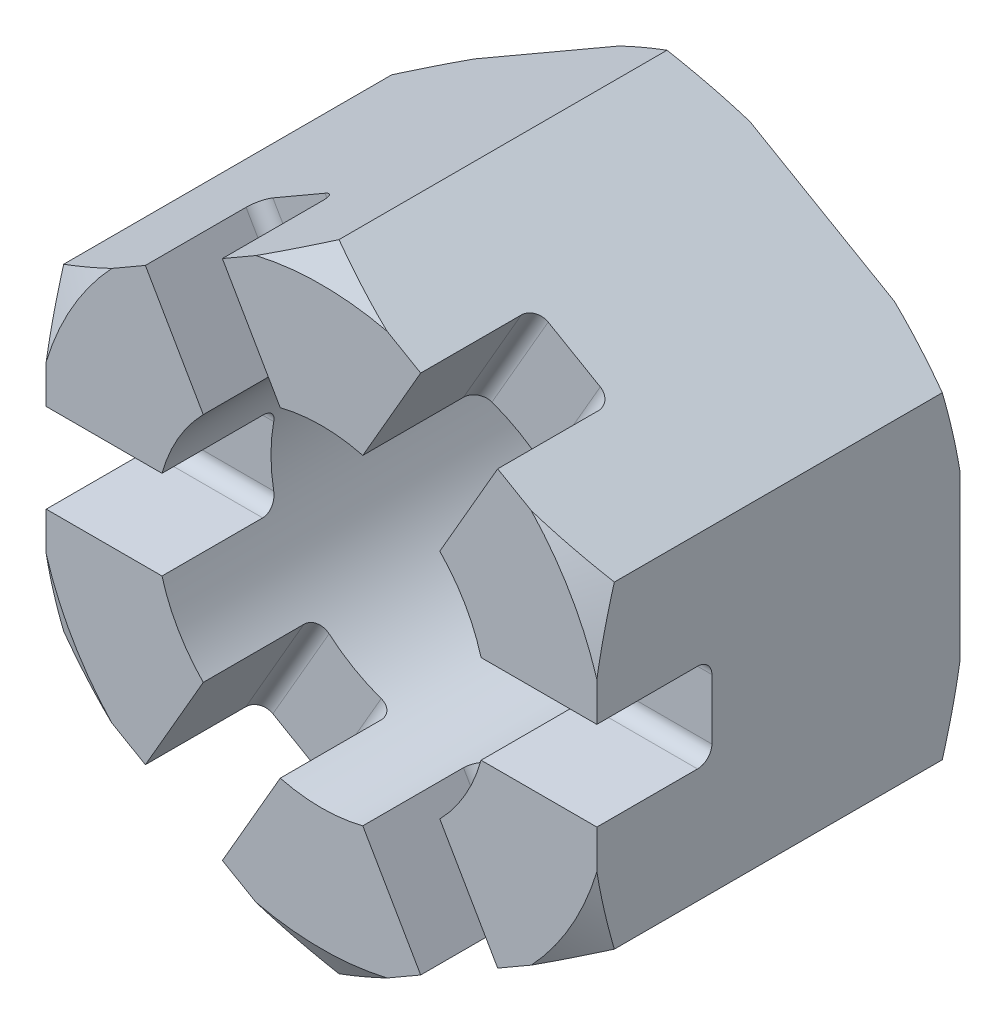
from build123d import *

# Parameters (mm, degrees)
SKETCH_1_R               = 15.835
EXTRUDE_848_DEPTH        = 34.7
SKETCH_2_OUTSIDE_W       = 259.61
SKETCH_2_OUTSIDE_H       = 267.754
SKETCH_2_OUTSIDE_R       = 27.5
CUT_EXTRUDE_1_DEPTH      = 54.111562242
CUT_EXTRUDE_1_DRAFT      = -60
SKETCH_3_OUTSIDE_W       = 259.61
SKETCH_3_OUTSIDE_H       = 267.754
SKETCH_3_OUTSIDE_R       = 27.5
CUT_EXTRUDE_2_DEPTH      = 54.111562242
CUT_EXTRUDE_2_DRAFT      = -60
CUT_EXTRUDE_3_DEPTH      = 70.9965292
PATTERN_CIRCULAR_1_COUNT = 3
CHAMFER_1_SIZE           = 0.576785714


with BuildPart() as part:
    # 草图1 → Extrude 848 (new body)
    with BuildSketch(Plane.XY):
        Polygon((0, 30.395), (-26.322842148, 15.1975), (-26.322842148, -15.1975), (0, -30.395), (26.322842148, -15.1975), (26.322842148, 15.1975), align=None)
        Circle(SKETCH_1_R, mode=Mode.SUBTRACT)
    extrude(amount=EXTRUDE_848_DEPTH)


with BuildPart() as cut_extrude_1_tool:
    # 草图2 outside → 切除-拉伸1 (with draft: the straight prism first)
    with BuildSketch(Plane(origin=(0, 0, 0), x_dir=(-1, 0, 0), z_dir=(0, 0, -1))):
        Rectangle(SKETCH_2_OUTSIDE_W, SKETCH_2_OUTSIDE_H)
        Circle(SKETCH_2_OUTSIDE_R, mode=Mode.SUBTRACT)
    extrude(amount=-CUT_EXTRUDE_1_DEPTH)
    # 切除-拉伸1: the draft: its side faces are tilted about the plane it starts from
    cut_extrude_1_sides = [cut_extrude_1_tool.faces().sort_by_distance(p)[0] for p in [
        (0, -133.877, 27.055781121),
        (-129.805, 0, 27.055781121),
        (0, 133.877, 27.055781121),
        (129.805, 0, 27.055781121),
        (27.5, 0, 27.055781121),
    ]]
    draft(cut_extrude_1_sides, Plane(origin=(0, 0, 0), x_dir=(-1, 0, 0), z_dir=(0, 0, -1)), CUT_EXTRUDE_1_DRAFT)


with BuildPart() as part_1:
    add(part.part)

    # 切除-拉伸1: cut by cut_extrude_1_tool
    add(cut_extrude_1_tool.part, mode=Mode.SUBTRACT)


with BuildPart() as cut_extrude_2_tool:
    # 草图3 outside → 切除-拉伸2 (with draft: the straight prism first)
    with BuildSketch(Plane.XY.offset(34.7)):
        Rectangle(SKETCH_3_OUTSIDE_W, SKETCH_3_OUTSIDE_H)
        Circle(SKETCH_3_OUTSIDE_R, mode=Mode.SUBTRACT)
    extrude(amount=-CUT_EXTRUDE_2_DEPTH)
    # 切除-拉伸2: the draft: its side faces are tilted about the plane it starts from
    cut_extrude_2_sides = [cut_extrude_2_tool.faces().sort_by_distance(p)[0] for p in [
        (0, -133.877, 7.644218879),
        (129.805, 0, 7.644218879),
        (0, 133.877, 7.644218879),
        (-129.805, 0, 7.644218879),
        (-27.5, 0, 7.644218879),
    ]]
    draft(cut_extrude_2_sides, Plane.XY.offset(34.7), CUT_EXTRUDE_2_DRAFT)


with BuildPart() as part_2:
    add(part_1.part)

    # 切除-拉伸2: cut by cut_extrude_2_tool
    add(cut_extrude_2_tool.part, mode=Mode.SUBTRACT)

    # 草图6 → 切除-拉伸3 (cut, through all)
    with BuildSketch(Plane(origin=(26.322842148, 0, 0), x_dir=(0, 0, -1), z_dir=(1, 0, 0))):
        with BuildLine():
            Line((-34.7, -4.25), (-34.7, 4.25))
            Line((-34.7, 4.25), (-25.075, 4.25))
            ThreePointArc((-25.075, 4.25), (-24.102728176, 3.847271824), (-23.7, 2.875))
            Line((-23.7, 2.875), (-23.7, -2.875))
            ThreePointArc((-23.7, -2.875), (-24.102728176, -3.847271824), (-25.075, -4.25))
            Line((-25.075, -4.25), (-34.7, -4.25))
        make_face()
    cut_extrude_3 = extrude(amount=-CUT_EXTRUDE_3_DEPTH, mode=Mode.SUBTRACT)

    # 阵列(圆周)1: 切除-拉伸3 ×3 about axis
    pattern_circular_1_axis = Axis((0, 0, 0), (0, 0, 1))
    for i in range(1, PATTERN_CIRCULAR_1_COUNT):
        add(cut_extrude_3.rotate(pattern_circular_1_axis, i * 360 / PATTERN_CIRCULAR_1_COUNT), mode=Mode.SUBTRACT)

    # 倒角1
    chamfer_1_edges = [part_2.edges().sort_by_distance(p)[0] for p in [
        (-15.835, 0, 0),
    ]]
    chamfer(chamfer_1_edges, length=CHAMFER_1_SIZE)


solid = part_2.part
